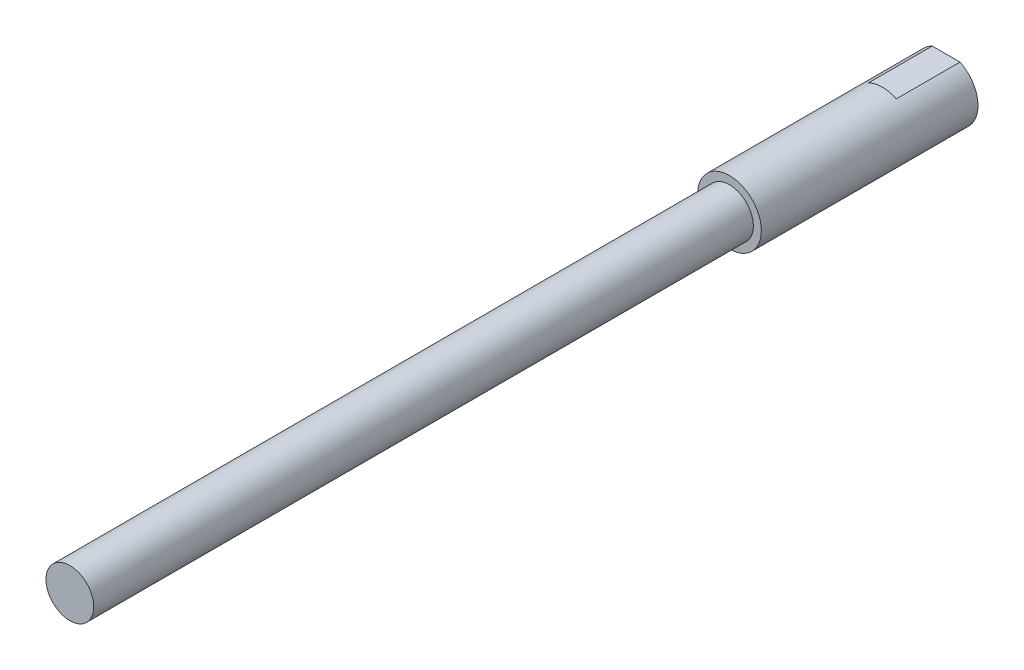
SolidWorks part; units mm, degrees
ref_plane "前视基准面" through (0, 0, 0) normal (0, 0, 1) x (1, 0, 0)
ref_plane "上视基准面" through (0, 0, 0) normal (0, 1, 0) x (1, 0, 0)
ref_plane "右视基准面" through (0, 0, 0) normal (1, 0, 0) x (0, 0, -1)
sketch "草图1" plane through (0, 0, 0) normal (0, 0, 1) x (1, 0, 0)
  circle A0 centre (0, 0) radius 7.5
  dimension "D1" = 15
extrude "凸台-拉伸1" add sketch "草图1" along normal blind 207
sketch "草图2" plane through (0, 0, 0) normal (0, 0, -1) x (-1, 0, 0)
  circle A0 centre (0, 0) radius 10
  dimension "D1" = 20
extrude "凸台-拉伸2" add sketch "草图2" along normal blind 68
sketch "草图3" plane through (0, 0, -68) normal (0, 0, -1) x (-1, 0, 0)
  line L1 (-11.5, -9) -> (11.5, -9)
  line L2 (-11.5, -9) -> (-11.5, 9)
  line L3 (-11.5, 9) -> (11.5, 9)
  line L4 (11.5, -9) -> (11.5, 9)
  line L5 (-11.5, -9) -> (11.5, 9) construction
  line L6 (-11.5, 9) -> (11.5, -9) construction
  point P0 (0, 0)
  dimension "D1" = 18
  dimension "D2" = 23
extrude "切除-拉伸1" cut sketch "草图3" against normal blind 20 flip side to cut
hole_wizard "M8 螺纹孔1" positions "3D草图1" profile "草图4" tap size "M8" standard "GB"
sketch3d "3D草图1"
  arc A0 (-4.3589, -9, -68) -> (-4.3589, 9, -68) centre (0, 0, -68) ccw construction
  point P0 (0, 0, -68)
  point P6 (0, 0, -78)
sketch "草图4" plane through (0, 0, -68) normal (1, 0, 0) x (0, 1, 0)
  line L0 (0, 0) -> (0, 20.2929)
  line L1 (0, 20.2929) -> (3.4, 18.25)
  line L2 (3.4, 18.25) -> (3.4, 0.625)
  line L3 (3.4, 0.625) -> (4.025, 0)
  line L5 (4.025, 0) -> (0, 0)
  line L6 (-3.4, 0.625) -> (-4.025, 0) construction
  line L10 (0, 20.2929) -> (-3.4, 18.25) construction
  line L11 (0, -6.35) -> (0, 107.95) construction
  dimension "螺纹孔钻头直径" = 6.8
  dimension "螺纹孔钻头深度" = 18.25
  dimension "近端锥形沉头孔直径" = 8.05
  dimension "近端锥形沉头孔角度" = 90
  dimension "导头角度" = 118
cosmetic thread "孔螺蚊线1" parameters "D1"=12, "D2"=8
